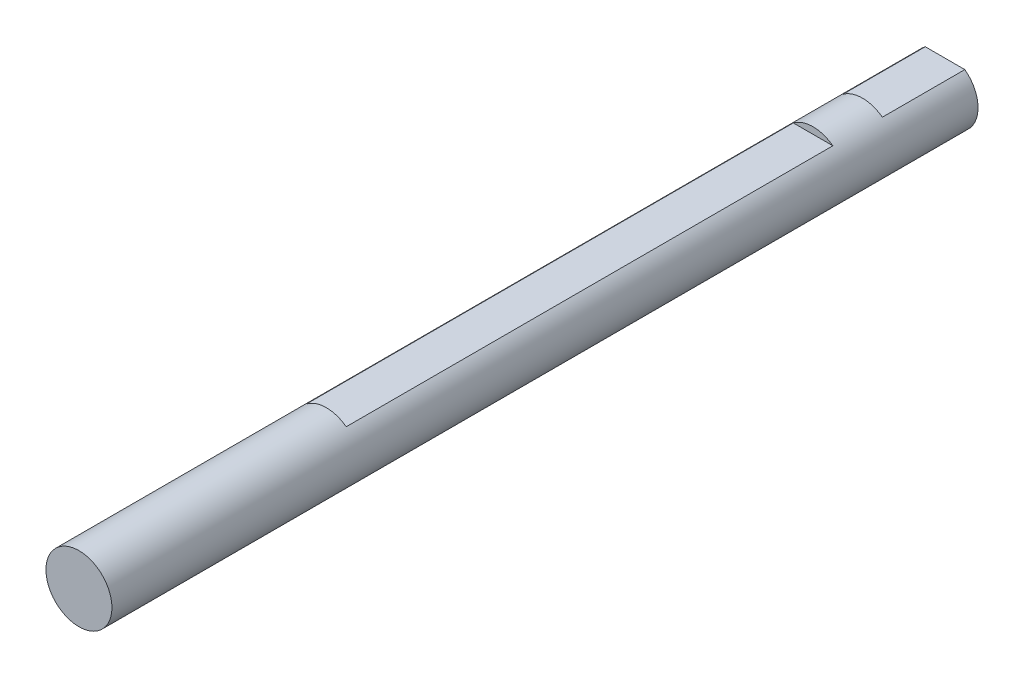
SolidWorks part; units mm, degrees
ref_plane "前视基准面" through (0, 0, 0) normal (0, 0, 1) x (1, 0, 0)
ref_plane "上视基准面" through (0, 0, 0) normal (0, 1, 0) x (1, 0, 0)
ref_plane "右视基准面" through (0, 0, 0) normal (1, 0, 0) x (0, 0, -1)
sketch "草图1" plane through (0, 0, 0) normal (0, 0, 1) x (1, 0, 0)
  circle A0 centre (-9.4959, 0) radius 4
  dimension "D1" = 8
extrude "凸台-拉伸1" add sketch "草图1" along normal blind 105
sketch "草图2" plane through (0, 0, 0) normal (0, 0, -1) x (-1, 0, 0)
  line L0 (7.0959, 3.2) -> (11.8959, 3.2)
  arc A0 (11.8959, 3.2) -> (7.0959, 3.2) centre (9.4959, 0) ccw
  dimension "D1" = 3.2
extrude "切除-拉伸1" cut sketch "草图2" against normal blind 10
ref_plane "基准面4" through (0, 0, 16) normal (0, 0, -1) x (-1, 0, 0)
sketch "草图3" plane through (0, 0, 16) normal (0, 0, -1) x (-1, 0, 0)
  line L0 (7.0959, 3.2) -> (11.8959, 3.2)
  arc A0 (11.8959, 3.2) -> (7.0959, 3.2) centre (9.4959, 0) ccw
extrude "切除-拉伸2" cut sketch "草图3" against normal blind 59
